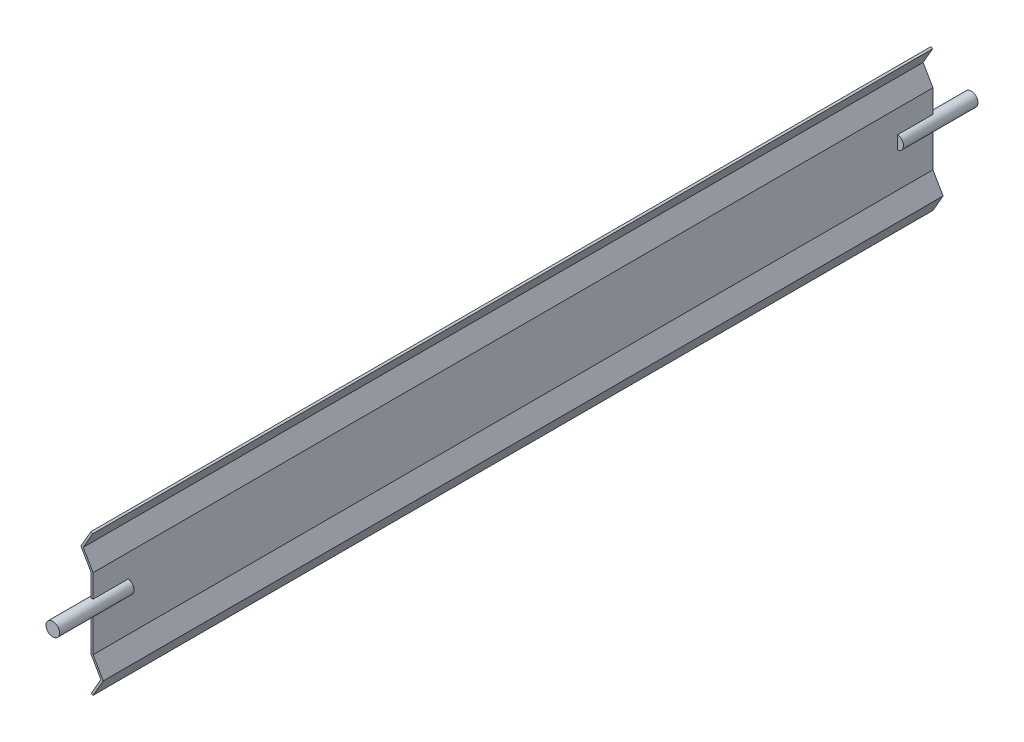
SolidWorks part; units mm, degrees
ref_plane "Front Plane" through (0, 0, 0) normal (0, 0, 1) x (1, 0, 0)
ref_plane "Top Plane" through (0, 0, 0) normal (0, 1, 0) x (1, 0, 0)
ref_plane "Right Plane" through (0, 0, 0) normal (1, 0, 0) x (0, 0, -1)
sketch "Sketch1" plane through (0, 0, 0) normal (0, 0, 1) x (1, 0, 0)
  line L0 (0, 0) -> (7.5, 12.9904)
  line L1 (7.5, 12.9904) -> (0, 25.9808)
  line L2 (0, 25.9808) -> (0, 78.4212)
  line L3 (0, 78.4212) -> (-7.2679, 91.0096)
  line L4 (-7.2679, 91.0096) -> (-0.201, 103.25)
  line L5 (-1.299, 0.75) -> (5.7679, 12.9904)
  line L6 (5.7679, 12.9904) -> (-1.5, 25.5788)
  line L7 (-1.5, 25.5788) -> (-1.5, 78.0192)
  line L8 (-1.5, 78.0192) -> (-9, 91.0096)
  line L9 (-9, 91.0096) -> (-1.5, 104)
  line L10 (-0.201, 103.25) -> (-1.5, 104)
  line L11 (0, 0) -> (-1.299, 0.75)
  dimension "D1" = 1.5
  dimension "D2" = 120
  dimension "D3" = 150
  dimension "D4" = 120
  dimension "D5" = 150
  dimension "D6" = 104
  dimension "D7" = 15
  dimension "D8" = 15
  dimension "D9" = 15
  dimension "D10" = 15
extrude "Boss-Extrude1" add sketch "Sketch1" along normal mid plane 620
sketch "Sketch2" plane through (0, 0, 310) normal (0, 0, 1) x (1, 0, 0)
  line L0 (-1.5, 56.5) -> (0, 56.5) construction
  line L1 (-1.5, 78.0192) -> (-1.5, 25.5788) construction
  line L2 (0, 25.9808) -> (0, 78.4212) construction
  circle A0 centre (-0.75, 56.5) radius 5
  dimension "D1" = 10
  dimension "D2" = 56.5
extrude "Boss-Extrude2" add sketch "Sketch2" along normal blind 29 and the other way blind 26
mirror "Mirror1" about plane through (0, 0, 0) normal (0, 0, 1) of "Boss-Extrude2"
